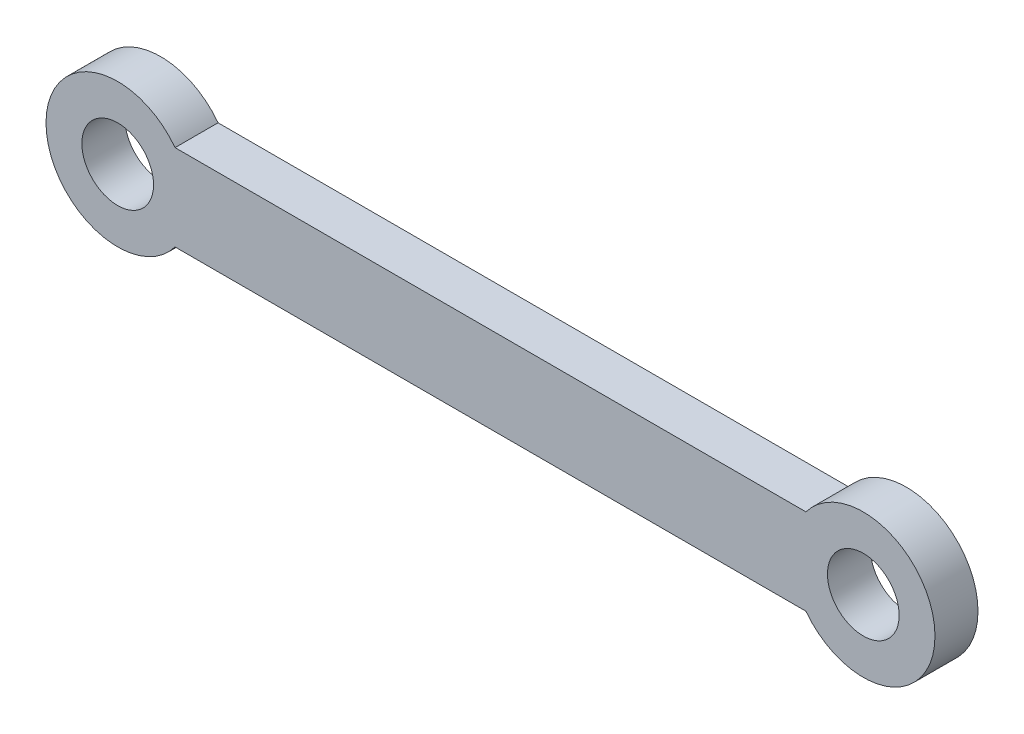
SolidWorks part; units mm, degrees
ref_plane "Front Plane" through (0, 0, 0) normal (0, 0, 1) x (1, 0, 0)
ref_plane "Top Plane" through (0, 0, 0) normal (0, 1, 0) x (1, 0, 0)
ref_plane "Right Plane" through (0, 0, 0) normal (1, 0, 0) x (0, 0, -1)
sketch "Sketch1" plane through (0, 0, 0) normal (0, 0, 1) x (1, 0, 0)
  line L2 (0, 0) -> (52, 0) construction
  line L3 (4, 3) -> (48, 3)
  line L4 (4, -3) -> (48, -3)
  circle A0 centre (0, 0) radius 2.5
  arc A1 (4, 3) -> (4, -3) centre (0, 0) ccw
  circle A2 centre (52, 0) radius 2.5
  arc A3 (48, -3) -> (48, 3) centre (52, 0) ccw
  dimension "D1" = 52
  dimension "D2" = 5
  dimension "D3" = 5
  dimension "D4" = 10
  dimension "D5" = 10
  dimension "D8" = 6
  dimension "D9" = 3
extrude "Boss-Extrude1" add sketch "Sketch1" along normal blind 3
